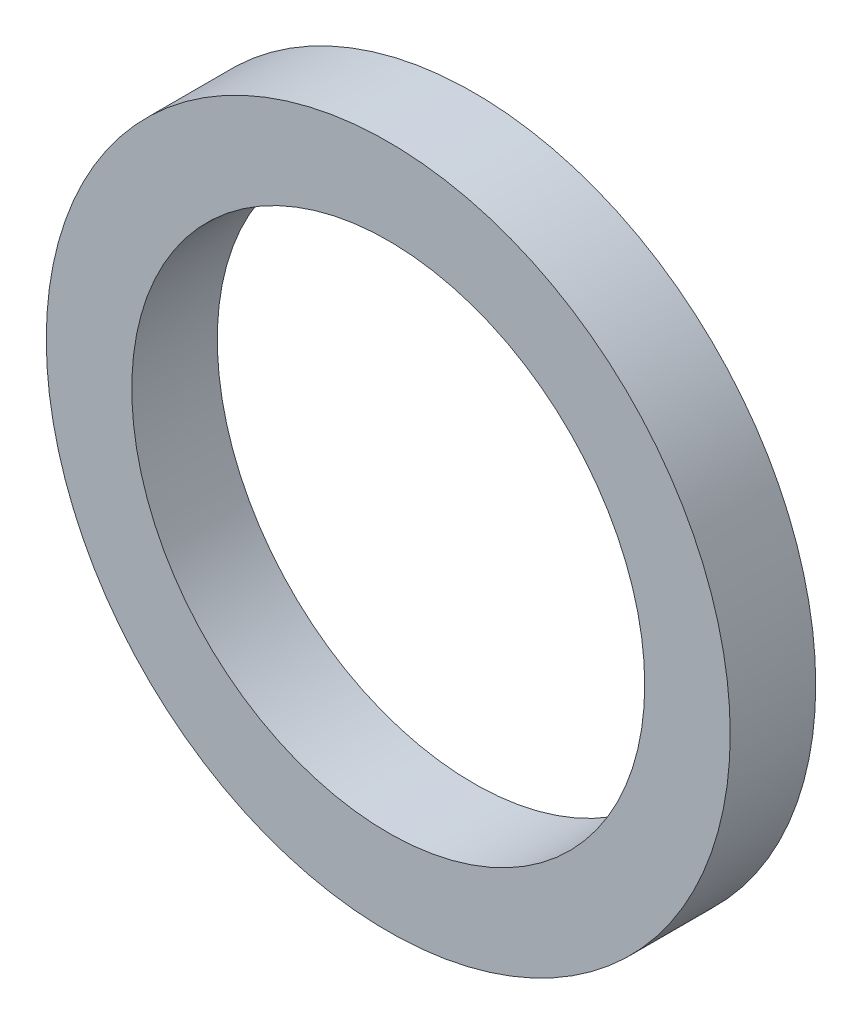
SolidWorks part; units mm, degrees
ref_plane "Front Plane" through (0, 0, 0) normal (0, 0, 1) x (1, 0, 0)
ref_plane "Top Plane" through (0, 0, 0) normal (0, 1, 0) x (1, 0, 0)
ref_plane "Right Plane" through (0, 0, 0) normal (1, 0, 0) x (0, 0, -1)
sketch "Sketch1" plane through (0, 0, 0) normal (0, 0, 1) x (1, 0, 0)
  circle A0 centre (0, 0) radius 4
  circle A1 centre (0, 0) radius 3
  dimension "D1" = 6
  dimension "D2" = 8
extrude "Boss-Extrude1" add sketch "Sketch1" along normal blind 1
